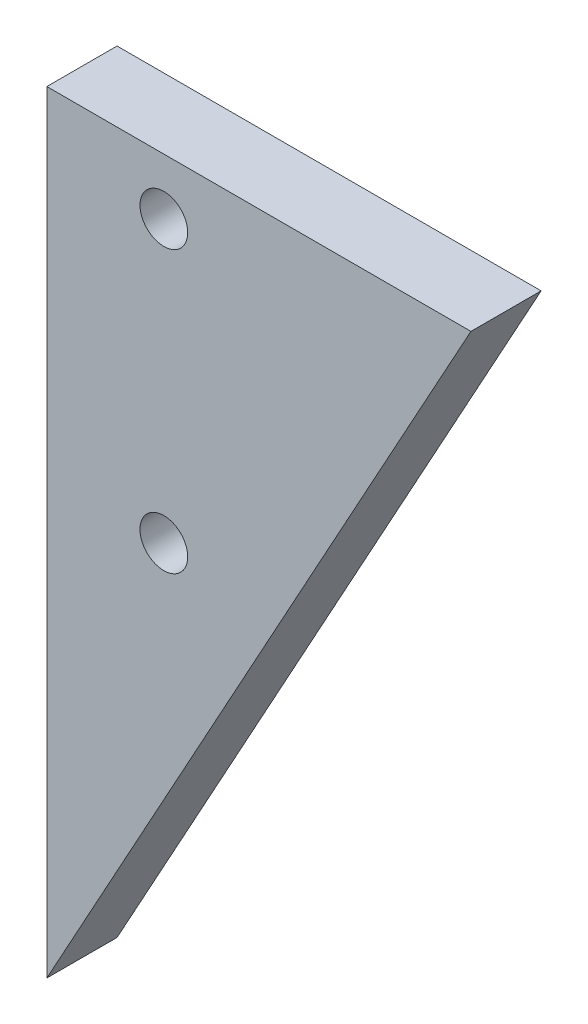
SolidWorks part; units mm, degrees
material "1023 碳钢板 (SS)"
ref_plane "Front Plane" through (0, 0, 0) normal (0, 0, 1) x (1, 0, 0)
ref_plane "Top Plane" through (0, 0, 0) normal (0, 1, 0) x (1, 0, 0)
ref_plane "Right Plane" through (0, 0, 0) normal (1, 0, 0) x (0, 0, -1)
sketch "Sketch1" plane through (0, 0, 0) normal (0, 0, 1) x (1, 0, 0)
  line L0 (0, 0) -> (-90.6345, 0)
  line L5 (-90.6345, 0) -> (-90.6345, -165)
  line L6 (-90.6345, -165) -> (0, 0)
  circle A0 centre (-65.6345, -12) radius 4.5
  circle A1 centre (-65.6345, -72) radius 4.5
  dimension "D5" = 9
  dimension "D6" = 25
  dimension "D1" = 61.22
  dimension "D2" = 165
  dimension "D3" = 12
  dimension "D4" = 60
extrude "Boss-Extrude2" add sketch "Sketch1" along normal blind 15
hole_wizard "M12 Tapped Hole1" positions "Sketch3" profile "Sketch4" tap size "M12" standard "ISO"
sketch "Sketch3" plane through (0, 0, 15) normal (0, 0, 1) x (1, 0, 0)
  point P0 (-65.6345, -12)
  point P3 (-65.6345, -72)
sketch "Sketch4" plane through (-65.6345, -12, 15) normal (1, 0, 0) x (0, -1, 0)
  line L0 (0, 0) -> (0, 32.3144)
  line L1 (0, 32.3144) -> (5.1, 29.25)
  line L2 (5.1, 29.25) -> (5.1, 0)
  line L5 (5.1, 0) -> (0, 0)
  line L10 (0, 32.3144) -> (-5.1, 29.25) construction
  line L11 (0, -6.35) -> (0, 107.95) construction
  dimension "螺纹孔钻头直径" = 10.2
  dimension "螺纹孔钻头深度" = 29.25
  dimension "导头角度" = 118
cosmetic thread "Hole Thread Line 1"
cosmetic thread "Hole Thread Line 2"
